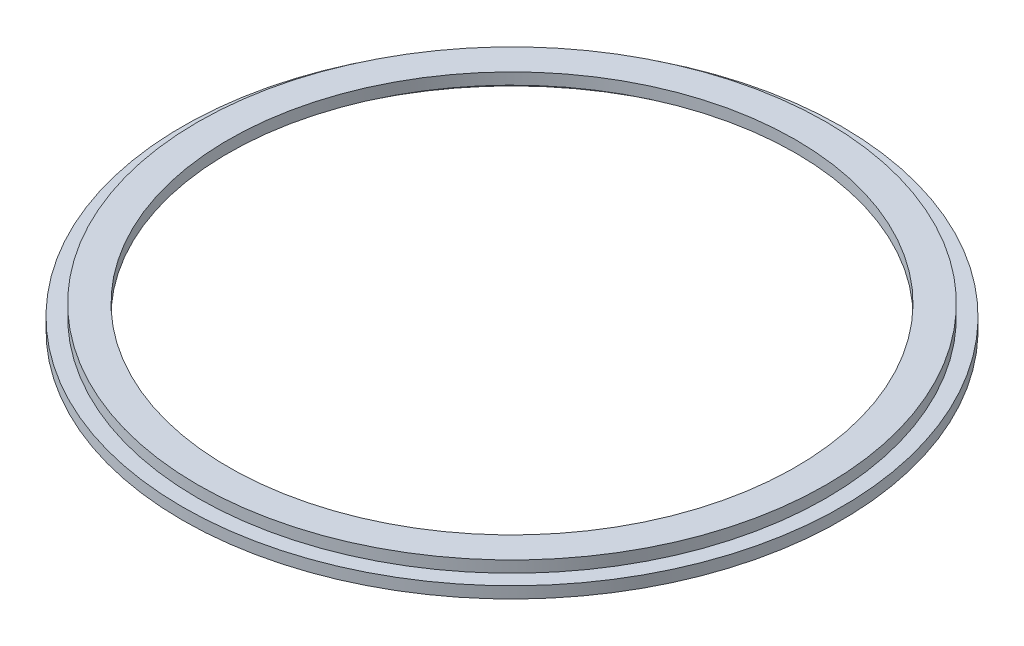
from build123d import *


with BuildPart() as part:
    # 草图1 → 旋转1 (revolve)
    with BuildSketch(Plane.XY, mode=Mode.PRIVATE) as revolve_1_sk:
        Polygon((-37, 0), (-41, 0), (-41, -1.5), (-43, -1.5), (-43, -3), (-39, -3), (-39, -1.5), (-37, -1.5), align=None)
    revolve(revolve_1_sk.sketch.rotate(Axis((0, 0, 0), (0, 1, 0)), 270), axis=Axis((0, 0, 0), (0, 1, 0)))


solid = part.part
